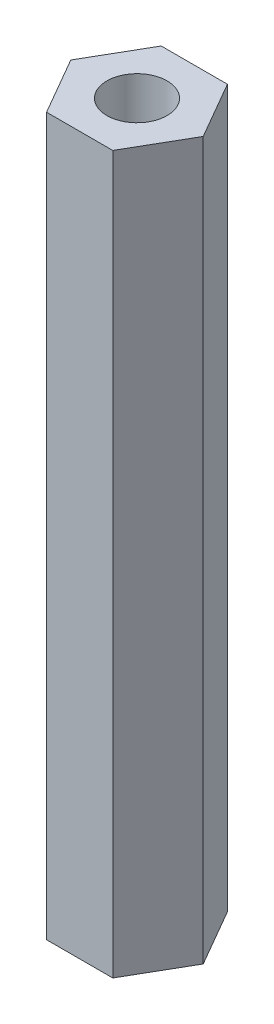
SolidWorks part; units mm, degrees
ref_plane "Front Plane" through (0, 0, 0) normal (0, 0, 1) x (1, 0, 0)
ref_plane "Top Plane" through (0, 0, 0) normal (0, 1, 0) x (1, 0, 0)
ref_plane "Right Plane" through (0, 0, 0) normal (1, 0, 0) x (0, 0, -1)
sketch "Sketch1" plane through (0, 0, 0) normal (0, 1, 0) x (1, 0, 0)
  line L1 (2.9329, -5.08) -> (5.8659, 0)
  line L2 (5.8659, 0) -> (2.9329, 5.08)
  line L3 (2.9329, 5.08) -> (-2.9329, 5.08)
  line L4 (-2.9329, 5.08) -> (-5.8659, 0)
  line L5 (-5.8659, 0) -> (-2.9329, -5.08)
  line L6 (-2.9329, -5.08) -> (2.9329, -5.08)
  circle A0 centre (0, 0) radius 5.08 construction
  dimension "D1" = 5.08
  dimension "D2" = 5.08
extrude "Boss-Extrude1" add sketch "Sketch1" along normal blind 63.5
sketch "Sketch2" plane through (0, 0, 0) normal (0, 1, 0) x (1, 0, 0)
  circle A0 centre (0, 0) radius 2.667
  dimension "D1" = 5.334
extrude "Cut-Extrude1" cut sketch "Sketch2" along normal blind 127
scale "Scale1" bodies to scale 102 scale about origin uniform scaling yes scale factor 2
